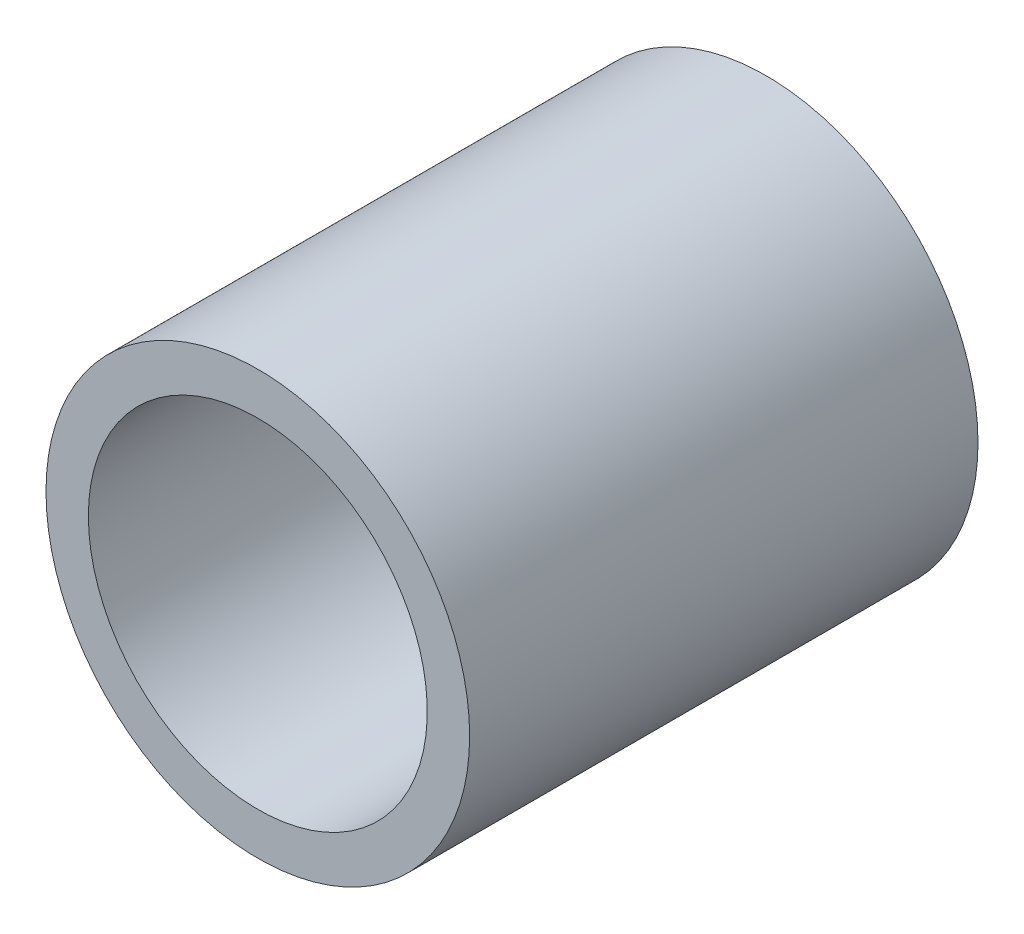
SolidWorks part; units mm, degrees
ref_plane "Front Plane" through (0, 0, 0) normal (0, 0, 1) x (1, 0, 0)
ref_plane "Top Plane" through (0, 0, 0) normal (0, 1, 0) x (1, 0, 0)
ref_plane "Right Plane" through (0, 0, 0) normal (1, 0, 0) x (0, 0, -1)
other "Configuration Table"
sketch "Sketch1" plane through (0, 0, 0) normal (0, 0, 1) x (1, 0, 0)
  circle A0 centre (0, 0) radius 60
  circle A1 centre (0, 0) radius 75
  dimension "D1" = 120
  dimension "D2" = 150
extrude "Boss-Extrude1" add sketch "Sketch1" along normal blind 180
